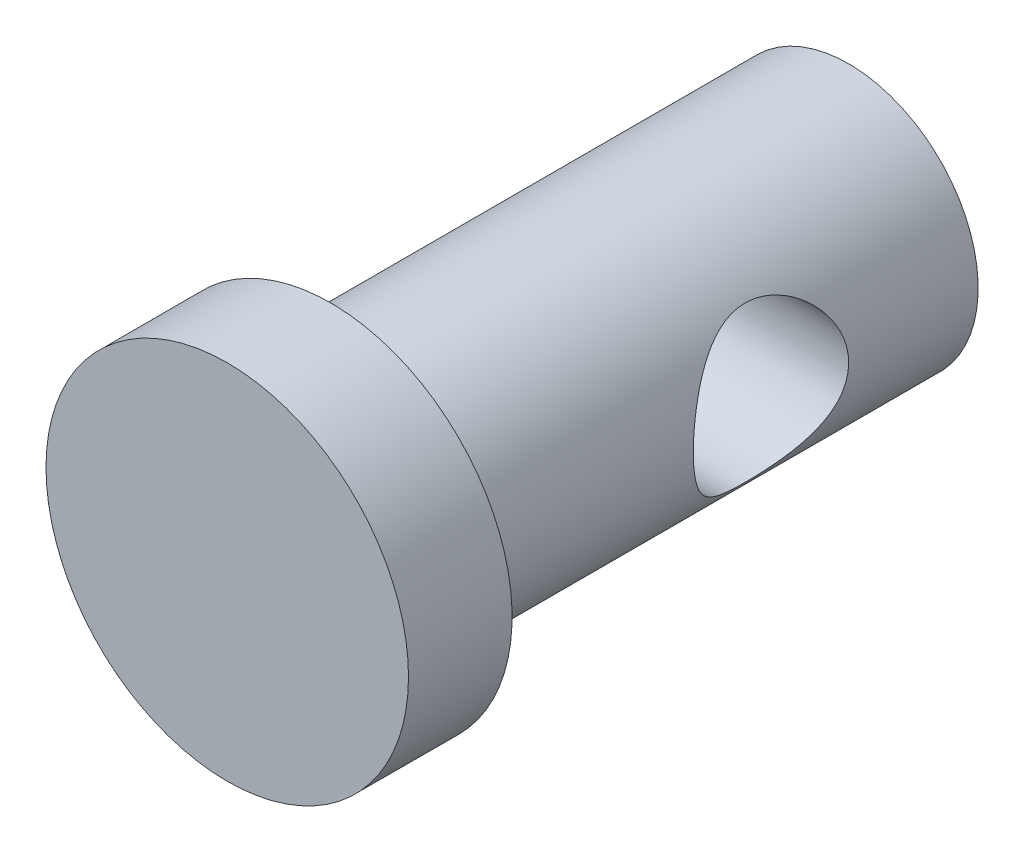
SolidWorks part; units mm, degrees
ref_plane "Front Plane" through (0, 0, 0) normal (0, 0, 1) x (1, 0, 0)
ref_plane "Top Plane" through (0, 0, 0) normal (0, 1, 0) x (1, 0, 0)
ref_plane "Right Plane" through (0, 0, 0) normal (1, 0, 0) x (0, 0, -1)
sketch "Sketch1" plane through (0, 0, 0) normal (0, 0, 1) x (1, 0, 0)
  circle A0 centre (0, 0) radius 17.5
  dimension "D1" = 35
extrude "Boss-Extrude1" add sketch "Sketch1" along normal blind 60
chamfer "Chamfer1" distance 1 angle 45 1 edges at (17.5, 0, 0)
sketch "Sketch2" plane through (0, 0, 0) normal (1, 0, 0) x (0, 0, -1)
  line L0 (-60, 17.5) -> (-60, -17.5) construction
  circle A0 centre (-20, 0) radius 7.5
  dimension "D2" = 15
  dimension "D1" = 40
extrude "Cut-Extrude1" cut sketch "Sketch2" against normal mid plane 60
sketch "Sketch3" plane through (0, 0, 0) normal (0, 0, -1) x (-1, 0, 0)
  circle A0 centre (0, 0) radius 12.5
  dimension "D1" = 25
extrude "Cut-Extrude2" cut sketch "Sketch3" against normal blind 50 flip side to cut
equation "\"A\"= \"代号代码\""
equation "\"B\"= \"名称代码\""
